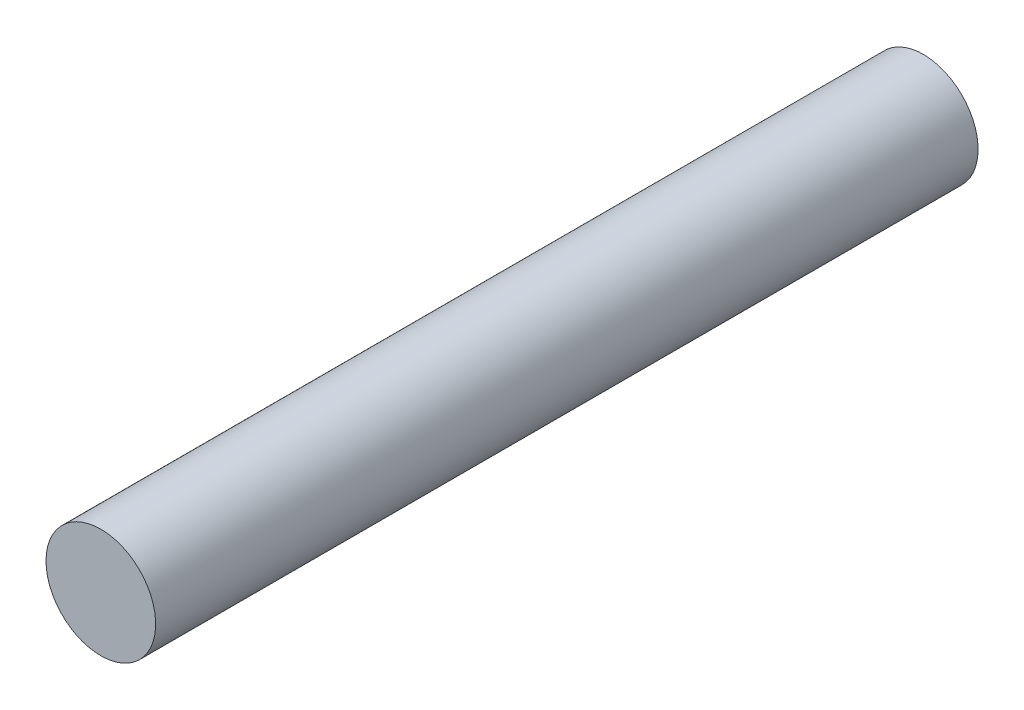
SolidWorks part; units mm, degrees
ref_plane "Front Plane" through (0, 0, 0) normal (0, 0, 1) x (1, 0, 0)
ref_plane "Top Plane" through (0, 0, 0) normal (0, 1, 0) x (1, 0, 0)
ref_plane "Right Plane" through (0, 0, 0) normal (1, 0, 0) x (0, 0, -1)
sketch "Sketch1" plane through (0, 0, 0) normal (0, 0, 1) x (1, 0, 0)
  circle A0 centre (0, 0) radius 3
  dimension "D1" = 6
extrude "Boss-Extrude1" add sketch "Sketch1" along normal mid plane 45
